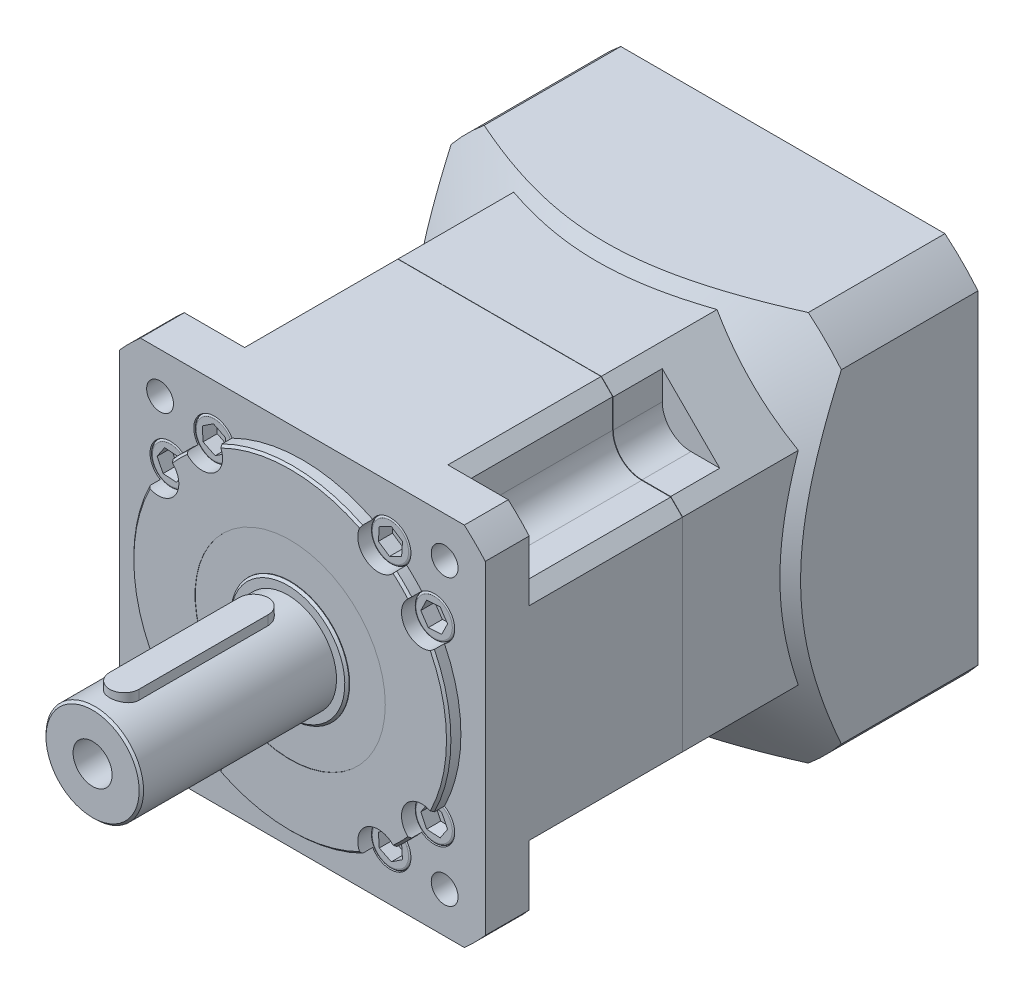
from build123d import *

# Parameters (mm, degrees)
EXTRUDE_START                    = 8
EXTRUDE_2_DEPTH                  = 15
CHAMFER_1_SIZE                   = 0.9
EXTRUDE_START_2                  = 42.45
SKETCH_6_W                       = 150
SKETCH_6_H                       = 150
EXTRUDE_1_DEPTH                  = 154.55
SKETCH_7_R                       = 5.5
CUT_EXTRUDE_1_DEPTH              = 18
CUT_EXTRUDE_START                = 179
CUT_EXTRUDE_3_DEPTH              = 136.55
CUT_EXTRUDE_2_DEPTH              = 83
CUT_EXTRUDE_4_DEPTH              = 62.8
PATTERN_CIRCULAR_1_COUNT         = 4
SKETCH_11_R                      = 8.4
CUT_EXTRUDE_5_DEPTH              = 5
CUT_EXTRUDE_START_2              = 197
SKETCH_12_R                      = 8.4
SKETCH_12_R_2                    = 8.25
CUT_EXTRUDE_6_DEPTH              = 9.9
CUT_EXTRUDE_7_DEPTH              = 5.775
FILLET_1_R                       = 0.825
PATTERN_CIRCULAR_2_COUNT         = 16
FILLET_1_OF_PATTERN_CIRCULAR_2_R = 0.825
CUT_EXTRUDE_START_3              = 201.9
SKETCH_14_R                      = 39
SKETCH_14_R_2                    = 24.3
CUT_EXTRUDE_8_DEPTH              = 0.1
EXTRUDE_3_DEPTH                  = 42.45
SKETCH_17_R                      = 4
CUT_EXTRUDE_9_DEPTH              = 24
PATTERN_CIRCULAR_3_COUNT         = 4
SKETCH_27_R                      = 150
CUT_EXTRUDE_15_DEPTH             = 96
SKETCH_21_R                      = 6.15
CUT_EXTRUDE_10_DEPTH             = 10
CUT_EXTRUDE_START_4              = 10
SKETCH_22_R                      = 6.15
SKETCH_22_R_2                    = 6
CUT_EXTRUDE_12_DEPTH             = 7.2
CUT_EXTRUDE_13_DEPTH             = 4.2
FILLET_2_R                       = 0.6
PATTERN_CIRCULAR_4_COUNT         = 4
FILLET_2_OF_PATTERN_CIRCULAR_4_R = 0.6
EXTRUDE_START_3                  = 10
EXTRUDE_4_DEPTH                  = 1
SKETCH_25_W                      = 150
SKETCH_25_H                      = 0.1
CUT_EXTRUDE_14_DEPTH             = 150


with BuildPart() as part:
    # 草图4 → 旋转1 (revolve)
    with BuildSketch(Plane(origin=(0, 0, 0), x_dir=(0, 0, -1), z_dir=(1, 0, 0))):
        Polygon((-202, 65), (-197, 65), (-197, 0), (-258.381197846, 0), (-263, 8), (-283, 8), (-283, 20), (-203, 20), (-203, 24.3), (-202, 24.3), align=None)
    revolve(axis=Axis((0, 0, 197), (0, 0, 1)))

    # 草图15 → 凸台-拉伸2 (add)
    with BuildSketch(Plane(origin=(0, 0, 0), x_dir=(1, 0, 0), z_dir=(0, 1, 0)).offset(EXTRUDE_START)):
        with BuildLine():
            Line((-6, -270), (-6, -217))
            ThreePointArc((-6, -217), (0, -211), (6, -217))
            Line((6, -217), (6, -270))
            ThreePointArc((6, -270), (0, -276), (-6, -270))
        make_face()
    extrude(amount=EXTRUDE_2_DEPTH)

    # 倒角1
    chamfer_1_edges = [part.edges().sort_by_distance(p)[0] for p in [
        (0, -65, 202),
        (0, -24.3, 203),
        (0, -20, 283),
    ]]
    chamfer(chamfer_1_edges, length=CHAMFER_1_SIZE)

    # 草图6 → 凸台-拉伸1 (add)
    with BuildSketch(Plane.XY.offset(EXTRUDE_START_2)):
        Rectangle(SKETCH_6_W, SKETCH_6_H)
    extrude(amount=EXTRUDE_1_DEPTH)

    # 草图7 → 切除-拉伸1 (cut)
    with BuildSketch(Plane.XY.offset(197)):
        with Locations((58.336309448, 58.336309448)):
            Circle(SKETCH_7_R)
        with BuildLine():
            Line((66.40732664, 75), (75, 75))
            Line((75, 75), (75, 66.40732664))
            ThreePointArc((75, 66.40732664), (70.834077362, 70.834077362), (66.40732664, 75))
        make_face()
    cut_extrude_1 = extrude(amount=-CUT_EXTRUDE_1_DEPTH, mode=Mode.SUBTRACT)

    # 草图9 → 切除-拉伸3 (cut)
    with BuildSketch(Plane.XY.offset(CUT_EXTRUDE_START)):
        Polygon((41.672618896, 75), (75, 41.672618896), (75, 75), align=None)
    cut_extrude_3 = extrude(amount=-CUT_EXTRUDE_3_DEPTH, mode=Mode.SUBTRACT)

    # 草图8 → 切除-拉伸2 (cut)
    with BuildSketch(Plane.XY.offset(CUT_EXTRUDE_START)):
        with BuildLine():
            Line((58.336309448, 46.553300859), (75, 46.553300859))
            Line((75, 46.553300859), (75, 75))
            Line((75, 75), (46.553300859, 75))
            Line((46.553300859, 75), (46.553300859, 58.336309448))
            ThreePointArc((46.553300859, 58.336309448), (50.004464172, 50.004464172), (58.336309448, 46.553300859))
        make_face()
    cut_extrude_2 = extrude(amount=-CUT_EXTRUDE_2_DEPTH, mode=Mode.SUBTRACT)

    # 草图10 → 切除-拉伸4 (cut)
    with BuildSketch(Plane(origin=(0, 0, 179), x_dir=(-1, 0, 0), z_dir=(0, 0, -1))):
        with BuildLine():
            Line((-46.553300859, 70.119318037), (-46.553300859, 58.336309448))
            ThreePointArc((-46.553300859, 58.336309448), (-50.004464172, 50.004464172), (-58.336309448, 46.553300859))
            Line((-58.336309448, 46.553300859), (-70.119318037, 46.553300859))
            Line((-70.119318037, 46.553300859), (-70.219318037, 46.453300859))
            Line((-70.219318037, 46.453300859), (-58.336309448, 46.453300859))
            ThreePointArc((-58.336309448, 46.453300859), (-49.933753494, 49.933753494), (-46.453300859, 58.336309448))
            Line((-46.453300859, 58.336309448), (-46.453300859, 70.219318037))
            Line((-46.453300859, 70.219318037), (-46.553300859, 70.119318037))
        make_face()
    cut_extrude_4 = extrude(amount=CUT_EXTRUDE_4_DEPTH, mode=Mode.SUBTRACT)

    # 阵列(圆周)1: 切除-拉伸1, 切除-拉伸3, 切除-拉伸2, 切除-拉伸4 ×4 about axis
    pattern_circular_1_axis = Axis((0, 0, 0), (0, 0, 1))
    add([cut_extrude_1.rotate(pattern_circular_1_axis, i * 360 / PATTERN_CIRCULAR_1_COUNT) for i in range(1, PATTERN_CIRCULAR_1_COUNT)], mode=Mode.SUBTRACT)
    add([cut_extrude_3.rotate(pattern_circular_1_axis, i * 360 / PATTERN_CIRCULAR_1_COUNT) for i in range(1, PATTERN_CIRCULAR_1_COUNT)], mode=Mode.SUBTRACT)
    add([cut_extrude_2.rotate(pattern_circular_1_axis, i * 360 / PATTERN_CIRCULAR_1_COUNT) for i in range(1, PATTERN_CIRCULAR_1_COUNT)], mode=Mode.SUBTRACT)
    add([cut_extrude_4.rotate(pattern_circular_1_axis, i * 360 / PATTERN_CIRCULAR_1_COUNT) for i in range(1, PATTERN_CIRCULAR_1_COUNT)], mode=Mode.SUBTRACT)

    # 草图11 → 切除-拉伸5 (cut)
    with BuildSketch(Plane.XY.offset(202)):
        with Locations((36.112065146, 54.0455248)):
            Circle(SKETCH_11_R)
    cut_extrude_5 = extrude(amount=-CUT_EXTRUDE_5_DEPTH, mode=Mode.SUBTRACT)

    # 草图12 → 切除-拉伸6 (cut)
    with BuildSketch(Plane.XY.offset(CUT_EXTRUDE_START_2)):
        with Locations((36.112065146, 54.0455248)):
            Circle(SKETCH_12_R)
        with Locations((36.112065146, 54.0455248)):
            Circle(SKETCH_12_R_2, mode=Mode.SUBTRACT)
    cut_extrude_6 = extrude(amount=-CUT_EXTRUDE_6_DEPTH, mode=Mode.SUBTRACT)

    # 草图13 → 切除-拉伸7 (cut)
    with BuildSketch(Plane.XY.offset(CUT_EXTRUDE_START_2)):
        Polygon((40.685148014, 50.989888518), (41.044865225, 56.478112596), (36.471782357, 59.533748877), (31.538982279, 57.101161081), (31.179265068, 51.612937003), (35.752347936, 48.557300722), align=None)
    cut_extrude_7 = extrude(amount=-CUT_EXTRUDE_7_DEPTH, mode=Mode.SUBTRACT)

    # 圆角1
    fillet_1_edges = [part.edges().sort_by_distance(p)[0] for p in [
        (27.862065146, 54.0455248, 197),
    ]]
    fillet(fillet_1_edges, radius=FILLET_1_R)

    # 阵列(圆周)2: 切除-拉伸5, 切除-拉伸6, 切除-拉伸7 ×16 about axis, 8 skipped
    pattern_circular_2_axis = Axis((0, 0, 0), (0, 0, -1))
    add([cut_extrude_5.rotate(pattern_circular_2_axis, i * 360 / PATTERN_CIRCULAR_2_COUNT) for i in range(1, PATTERN_CIRCULAR_2_COUNT) if i not in (2, 3, 6, 7, 10, 11, 14, 15)], mode=Mode.SUBTRACT)
    add([cut_extrude_6.rotate(pattern_circular_2_axis, i * 360 / PATTERN_CIRCULAR_2_COUNT) for i in range(1, PATTERN_CIRCULAR_2_COUNT) if i not in (2, 3, 6, 7, 10, 11, 14, 15)], mode=Mode.SUBTRACT)
    add([cut_extrude_7.rotate(pattern_circular_2_axis, i * 360 / PATTERN_CIRCULAR_2_COUNT) for i in range(1, PATTERN_CIRCULAR_2_COUNT) if i not in (2, 3, 6, 7, 10, 11, 14, 15)], mode=Mode.SUBTRACT)

    # 圆角1 of 阵列(圆周)2
    fillet_1_of_pattern_circular_2_edges = [part.edges().sort_by_distance(p)[0] for p in [
        (46.423518656, 39.269203463, 197),
        (54.0455248, -27.862065146, 197),
        (39.269203463, -46.423518656, 197),
        (-27.862065146, -54.0455248, 197),
        (-46.423518656, -39.269203463, 197),
        (-54.0455248, 27.862065146, 197),
        (-39.269203463, 46.423518656, 197),
    ]]
    fillet(fillet_1_of_pattern_circular_2_edges, radius=FILLET_1_OF_PATTERN_CIRCULAR_2_R)

    # 草图14 → 切除-拉伸8 (cut)
    with BuildSketch(Plane.XY.offset(CUT_EXTRUDE_START_3)):
        Circle(SKETCH_14_R)
        Circle(SKETCH_14_R_2, mode=Mode.SUBTRACT)
    extrude(amount=CUT_EXTRUDE_8_DEPTH, mode=Mode.SUBTRACT)

    # 草图16 → 凸台-拉伸3 (add)
    with BuildSketch(Plane.XY):
        with BuildLine():
            Line((80, -66.452990903), (80, 66.452990903))
            ThreePointArc((80, 66.452990903), (73.539105243, 73.539105243), (66.452990903, 80))
            Line((66.452990903, 80), (-66.452990903, 80))
            ThreePointArc((-66.452990903, 80), (-73.539105243, 73.539105243), (-80, 66.452990903))
            Line((-80, 66.452990903), (-80, -66.452990903))
            ThreePointArc((-80, -66.452990903), (-73.539105243, -73.539105243), (-66.452990903, -80))
            Line((-66.452990903, -80), (66.452990903, -80))
            ThreePointArc((66.452990903, -80), (73.539105243, -73.539105243), (80, -66.452990903))
        make_face()
    extrude(amount=EXTRUDE_3_DEPTH)

    # 草图17 → 切除-拉伸9 (cut)
    with BuildSketch(Plane.XY):
        with Locations((51.265241636, 51.265241636)):
            Circle(SKETCH_17_R)
    cut_extrude_9 = extrude(amount=CUT_EXTRUDE_9_DEPTH, mode=Mode.SUBTRACT)

    # 阵列(圆周)3: 切除-拉伸9 ×4 about axis
    pattern_circular_3_axis = Axis((0, 0, 0), (0, 0, 1))
    for i in range(1, PATTERN_CIRCULAR_3_COUNT):
        add(cut_extrude_9.rotate(pattern_circular_3_axis, i * 360 / PATTERN_CIRCULAR_3_COUNT), mode=Mode.SUBTRACT)

    # 草图26 → 旋转2 (revolve)
    with BuildSketch(Plane(origin=(0, 0, 0), x_dir=(0, 0, -1), z_dir=(1, 0, 0)), mode=Mode.PRIVATE) as revolve_2_sk:
        Polygon((-24, 150), (-24, 0), (-128.401591251, 0), align=None)
    revolve(revolve_2_sk.sketch.rotate(Axis((0, 0, 128.401591251), (0, 0, -1)), 180), axis=Axis((0, 0, 128.401591251), (0, 0, -1)))

    # 草图27 → 切除-拉伸15 (cut)
    with BuildSketch(Plane(origin=(0, 0, 0), x_dir=(-1, 0, 0), z_dir=(0, 0, -1))):
        Circle(SKETCH_27_R)
        with BuildLine():
            Line((-66.452990903, 80), (66.452990903, 80))
            ThreePointArc((66.452990903, 80), (73.539105243, 73.539105243), (80, 66.452990903))
            Line((80, 66.452990903), (80, -66.452990903))
            ThreePointArc((80, -66.452990903), (73.539105243, -73.539105243), (66.452990903, -80))
            Line((66.452990903, -80), (-66.452990903, -80))
            ThreePointArc((-66.452990903, -80), (-73.539105243, -73.539105243), (-80, -66.452990903))
            Line((-80, -66.452990903), (-80, 66.452990903))
            ThreePointArc((-80, 66.452990903), (-73.539105243, 73.539105243), (-66.452990903, 80))
        make_face(mode=Mode.SUBTRACT)
    extrude(amount=-CUT_EXTRUDE_15_DEPTH, mode=Mode.SUBTRACT)

    # 草图20 → 切除-旋转1 (revolve, cut)
    with BuildSketch(Plane(origin=(0, 0, 0), x_dir=(0, 0, -1), z_dir=(1, 0, 0)), mode=Mode.PRIVATE) as cut_revolve_1_sk:
        Polygon((0, 55), (-10, 55), (-10, 11), (-62, 11), (-62, 0), (0, 0), align=None)
    revolve(cut_revolve_1_sk.sketch.rotate(Axis((0, 0, 0), (0, 0, 1)), 180), axis=Axis((0, 0, 0), (0, 0, 1)), mode=Mode.SUBTRACT)

    # 草图21 → 切除-拉伸10 (cut)
    with BuildSketch(Plane.XY):
        with Locations((-21.04758878, 50.813374288)):
            Circle(SKETCH_21_R)
    cut_extrude_10 = extrude(amount=CUT_EXTRUDE_10_DEPTH, mode=Mode.SUBTRACT)

    # 草图22 → 切除-拉伸12 (cut)
    with BuildSketch(Plane.XY.offset(CUT_EXTRUDE_START_4)):
        with Locations(Location((-21.04758878, 50.813374288, 0), (0, 0, 205.705026153))):
            Circle(SKETCH_22_R)
        with Locations((-21.04758878, 50.813374288)):
            Circle(SKETCH_22_R_2, mode=Mode.SUBTRACT)
    cut_extrude_12 = extrude(amount=CUT_EXTRUDE_12_DEPTH, mode=Mode.SUBTRACT)

    # 草图23 → 切除-拉伸13 (cut)
    with BuildSketch(Plane.XY.offset(CUT_EXTRUDE_START_4)):
        Polygon((-20.525484011, 54.779153734), (-24.221002141, 53.248420004), (-24.74310691, 49.282640559), (-21.569693549, 46.847594843), (-17.874175419, 48.378328572), (-17.35207065, 52.344108018), align=None)
    cut_extrude_13 = extrude(amount=CUT_EXTRUDE_13_DEPTH, mode=Mode.SUBTRACT)

    # 圆角2
    fillet_2_edges = [part.edges().sort_by_distance(p)[0] for p in [
        (-27.04758878, 50.813374288, 10),
    ]]
    fillet(fillet_2_edges, radius=FILLET_2_R)

    # 阵列(圆周)4: 切除-拉伸10, 切除-拉伸12, 切除-拉伸13 ×4 about axis
    pattern_circular_4_axis = Axis((0, 0, 0), (0, 0, 1))
    add([cut_extrude_10.rotate(pattern_circular_4_axis, i * 360 / PATTERN_CIRCULAR_4_COUNT) for i in range(1, PATTERN_CIRCULAR_4_COUNT)], mode=Mode.SUBTRACT)
    add([cut_extrude_12.rotate(pattern_circular_4_axis, i * 360 / PATTERN_CIRCULAR_4_COUNT) for i in range(1, PATTERN_CIRCULAR_4_COUNT)], mode=Mode.SUBTRACT)
    add([cut_extrude_13.rotate(pattern_circular_4_axis, i * 360 / PATTERN_CIRCULAR_4_COUNT) for i in range(1, PATTERN_CIRCULAR_4_COUNT)], mode=Mode.SUBTRACT)

    # 圆角2 of 阵列(圆周)4
    fillet_2_of_pattern_circular_4_edges = [part.edges().sort_by_distance(p)[0] for p in [
        (-50.813374288, -27.04758878, 10),
        (27.04758878, -50.813374288, 10),
        (50.813374288, 27.04758878, 10),
    ]]
    fillet(fillet_2_of_pattern_circular_4_edges, radius=FILLET_2_OF_PATTERN_CIRCULAR_4_R)

    # 草图24 → 凸台-拉伸4 (add)
    with BuildSketch(Plane.XY.offset(EXTRUDE_START_3)):
        with BuildLine():
            Line((0.25, 32.999053017), (0.25, 10.997158724))
            ThreePointArc((0.25, 10.997158724), (11, 0), (0.25, -10.997158724))
            Line((0.25, -10.997158724), (0.25, -32.999053017))
            ThreePointArc((0.25, -32.999053017), (33, 0), (0.25, 32.999053017))
        make_face()
        with BuildLine():
            Line((-0.25, 32.999053017), (-0.25, 10.997158724))
            ThreePointArc((-0.25, 10.997158724), (-11, 0), (-0.25, -10.997158724))
            Line((-0.25, -10.997158724), (-0.25, -32.999053017))
            ThreePointArc((-0.25, -32.999053017), (-33, 0), (-0.25, 32.999053017))
        make_face()
    extrude(amount=-EXTRUDE_4_DEPTH)

    # 草图25 → 切除-拉伸14 (cut)
    with BuildSketch(Plane(origin=(0, 75, 0), x_dir=(1, 0, 0), z_dir=(0, 1, 0))):
        with Locations((0, -116.15)):
            Rectangle(SKETCH_25_W, SKETCH_25_H)
    extrude(amount=-CUT_EXTRUDE_14_DEPTH, mode=Mode.SUBTRACT)


with BuildPart() as cut_extrude_14_piece_1:
    # of the separate pieces the step leaves, piece 1, a body of its own (cut_extrude_14_pieces)
    add(part.part.solids().sort_by_distance((-50.813374288, -15.04758878, 10.6))[0])


with BuildPart() as cut_extrude_14_piece_2:
    # of the separate pieces the step leaves, piece 2, a body of its own (cut_extrude_14_pieces)
    add(part.part.solids().sort_by_distance((-41.672618896, -75, 116.2))[0])


solid = Compound([cut_extrude_14_piece_1.part, cut_extrude_14_piece_2.part])
